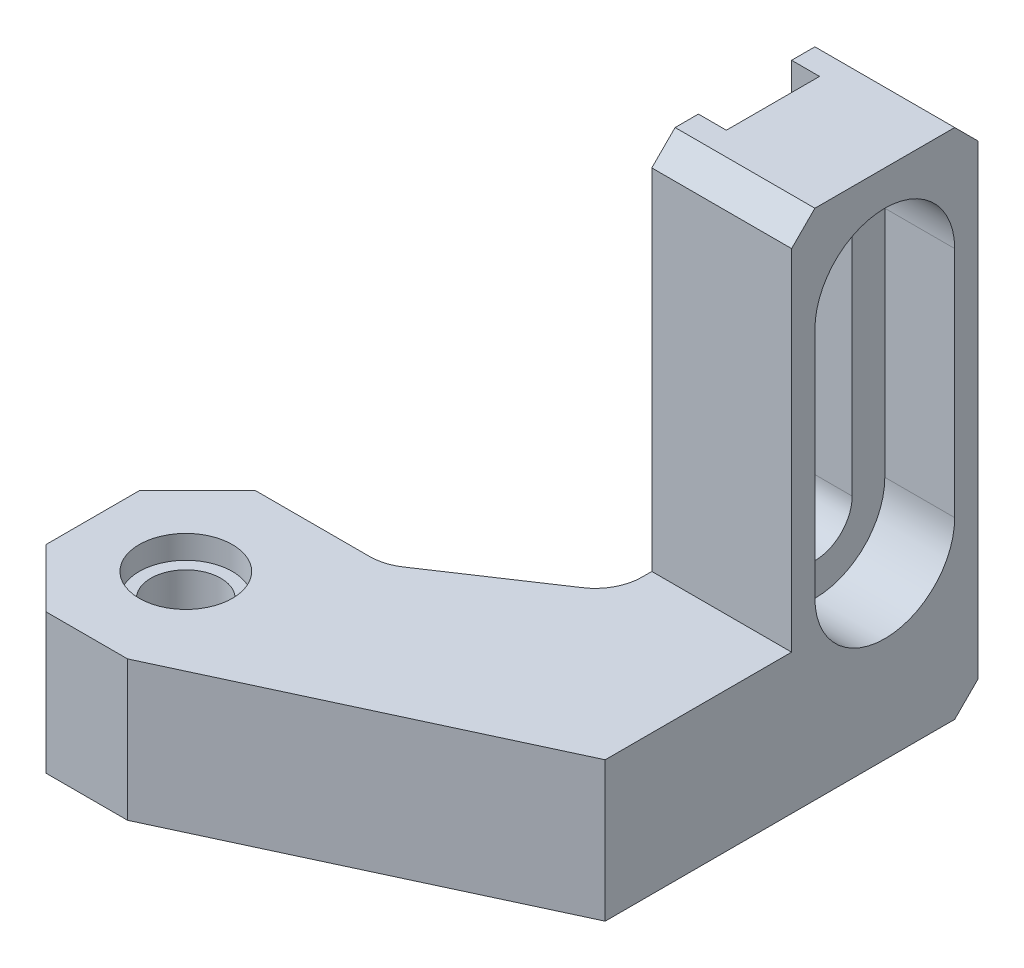
from build123d import *

# Parameters (mm, degrees)
SKETCH1_W           = 20
SKETCH1_H           = 22
BOSS_EXTRUDE1_DEPTH = 8
SKETCH2_W           = 20
SKETCH2_H           = 6
BOSS_EXTRUDE2_DEPTH = 14.5
SKETCH4_R           = 3.25
CUT_EXTRUDE2_DEPTH  = 5
SKETCH5_R           = 3.25
SKETCH5_R_2         = 1.5
BOSS_EXTRUDE3_DEPTH = 5
SKETCH6_W           = 14
SKETCH6_H           = 13.5
CUT_EXTRUDE3_DEPTH  = 34.018933962
SKETCH7_W           = 4
SKETCH7_H           = 22
CUT_EXTRUDE4_DEPTH  = 1.2
CUT_EXTRUDE5_DEPTH  = 34.018933962
CUT_EXTRUDE6_DEPTH  = 33.050741021
CUT_EXTRUDE7_DEPTH  = 3
CHAMFER3_SIZE       = 2.5
CHAMFER4_SIZE       = 1
BOSS_EXTRUDE4_DEPTH = 6
FILLET2_R           = 2
SKETCH14_R          = 1.5
CUT_EXTRUDE8_DEPTH  = 34.018933962
SKETCH15_R          = 2
CUT_EXTRUDE9_DEPTH  = 1


with BuildPart() as part:
    # Sketch1 → Boss-Extrude1 (new body)
    with BuildSketch(Plane.XY):
        Rectangle(SKETCH1_W, SKETCH1_H)
    extrude(amount=BOSS_EXTRUDE1_DEPTH)

    # Sketch2 → Boss-Extrude2 (add)
    with BuildSketch(Plane.XY.offset(8)):
        with Locations((0, -8)):
            Rectangle(SKETCH2_W, SKETCH2_H)
    extrude(amount=BOSS_EXTRUDE2_DEPTH)

    # Sketch4 → Cut-Extrude2 (cut)
    with BuildSketch(Plane(origin=(0, -11, 0), x_dir=(1, 0, 0), z_dir=(0, 1, 0))):
        with Locations(Location((-6, -18, 0), (0, 0, 90))):
            Circle(SKETCH4_R)
    extrude(amount=CUT_EXTRUDE2_DEPTH, mode=Mode.SUBTRACT)

    # Sketch6 → Cut-Extrude3 (cut, through all)
    with BuildSketch(Plane.XZ.offset(11)):
        with Locations((-3, 6.75)):
            Rectangle(SKETCH6_W, SKETCH6_H)
    extrude(amount=-CUT_EXTRUDE3_DEPTH, mode=Mode.SUBTRACT)

    # Sketch7 → Cut-Extrude4 (cut)
    with BuildSketch(Plane.ZY.offset(-4)):
        with Locations((4, 0)):
            Rectangle(SKETCH7_W, SKETCH7_H)
    extrude(amount=-CUT_EXTRUDE4_DEPTH, mode=Mode.SUBTRACT)

    # Sketch8 → Cut-Extrude5 (cut, through all)
    with BuildSketch(Plane.XZ.offset(11)):
        Polygon((-4, 22.5), (10, 16), (10, 22.5), align=None)
    extrude(amount=-CUT_EXTRUDE5_DEPTH, mode=Mode.SUBTRACT)

    # Sketch11 → Cut-Extrude6 (cut, through all)
    with BuildSketch(Plane(origin=(10, 0, 0), x_dir=(0, 0, -1), z_dir=(1, 0, 0))):
        with BuildLine():
            Line((-5.6, -3.5), (-5.6, 6.5))
            ThreePointArc((-5.6, 6.5), (-4, 8.1), (-2.4, 6.5))
            Line((-2.4, 6.5), (-2.4, -3.5))
            ThreePointArc((-2.4, -3.5), (-4, -5.1), (-5.6, -3.5))
        make_face()
    extrude(amount=-CUT_EXTRUDE6_DEPTH, mode=Mode.SUBTRACT)

    # Sketch12 → Cut-Extrude7 (cut)
    with BuildSketch(Plane(origin=(10, 0, 0), x_dir=(0, 0, -1), z_dir=(1, 0, 0))):
        with BuildLine():
            Line((-7, -3.5), (-7, 6.5))
            ThreePointArc((-7, 6.5), (-4, 9.5), (-1, 6.5))
            Line((-1, 6.5), (-1, -3.5))
            ThreePointArc((-1, -3.5), (-4, -6.5), (-7, -3.5))
        make_face()
    extrude(amount=-CUT_EXTRUDE7_DEPTH, mode=Mode.SUBTRACT)

    # Chamfer3
    chamfer3_edges = [part.edges().sort_by_distance(p)[0] for p in [
        (-10, -8, 22.5),
        (-10, -8, 13.5),
    ]]
    chamfer(chamfer3_edges, length=CHAMFER3_SIZE)

    # Chamfer4
    chamfer4_edges = [part.edges().sort_by_distance(p)[0] for p in [
        (7, -11, 0),
        (7, 11, 0),
        (7, 11, 8),
    ]]
    chamfer(chamfer4_edges, length=CHAMFER4_SIZE)

    # Sketch13 → Boss-Extrude4 (add)
    with BuildSketch(Plane.XZ.offset(11)):
        Polygon((-2, 13.5), (4, 9.5), (4, 13.5), align=None)
    extrude(amount=-BOSS_EXTRUDE4_DEPTH)

    # Fillet2
    fillet2_edges = [part.edges().sort_by_distance(p)[0] for p in [
        (-2, -8, 13.5),
        (4, -8, 9.5),
    ]]
    fillet(fillet2_edges, radius=FILLET2_R)

    # Sketch14 → Cut-Extrude8 (cut, through all)
    with BuildSketch(Plane.XZ.offset(11)):
        with Locations(Location((-6, 18, 0), (0, 0, 270))):
            Circle(SKETCH14_R)
    extrude(amount=-CUT_EXTRUDE8_DEPTH, mode=Mode.SUBTRACT)

    # Sketch15 → Cut-Extrude9 (cut)
    with BuildSketch(Plane(origin=(0, -5, 0), x_dir=(1, 0, 0), z_dir=(0, 1, 0))):
        with Locations(Location((-6, -18, 0), (0, 0, 270))):
            Circle(SKETCH15_R)
    extrude(amount=-CUT_EXTRUDE9_DEPTH, mode=Mode.SUBTRACT)


with BuildPart() as body_2:
    # Sketch5 → Boss-Extrude3 (new body)
    with BuildSketch(Plane(origin=(0, -11, 0), x_dir=(1, 0, 0), z_dir=(0, 1, 0))):
        with Locations(Location((-6, -18, 0), (0, 0, 90))):
            Circle(SKETCH5_R)
        with Locations(Location((-6, -18, 0), (0, 0, 90))):
            Circle(SKETCH5_R_2, mode=Mode.SUBTRACT)
    extrude(amount=BOSS_EXTRUDE3_DEPTH)


solid = Compound([part.part, body_2.part])
